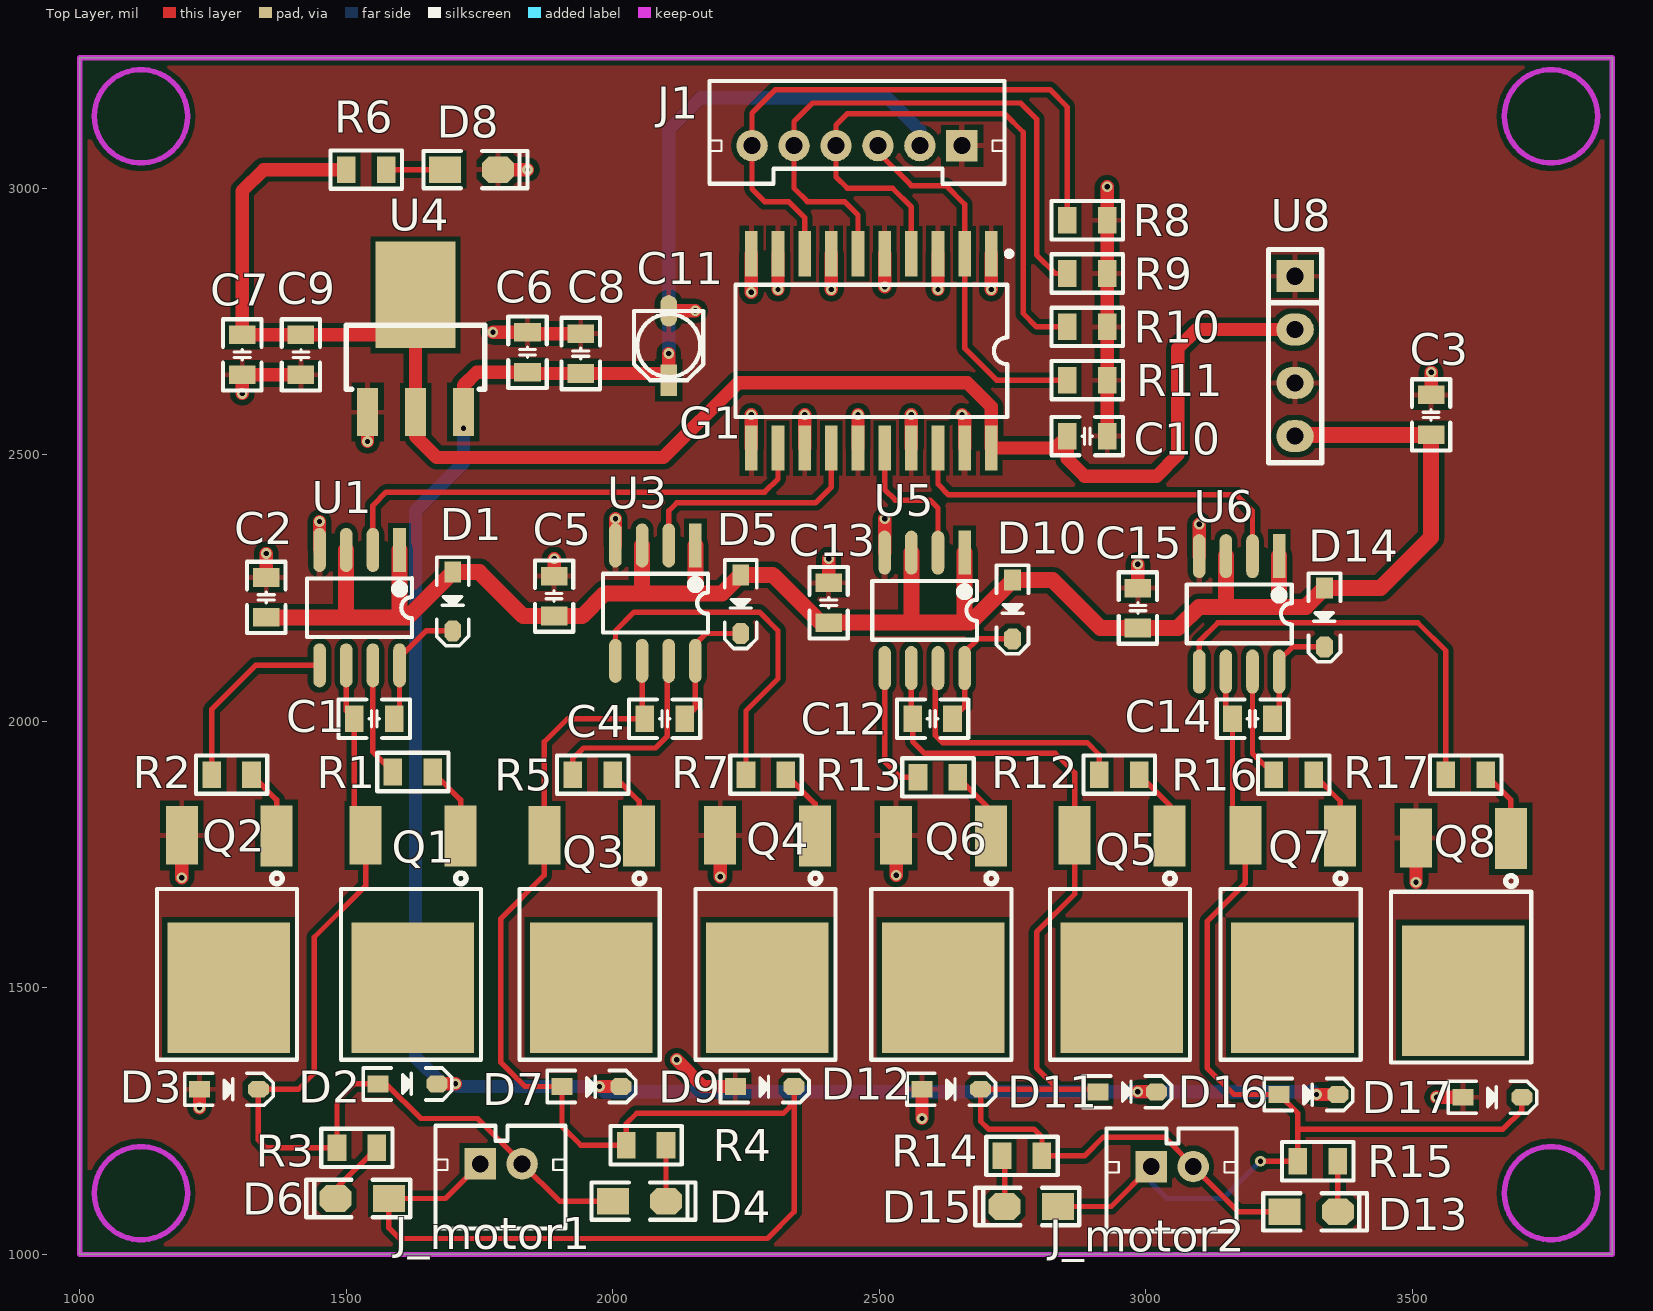
[diagram p0: Top Layer view]
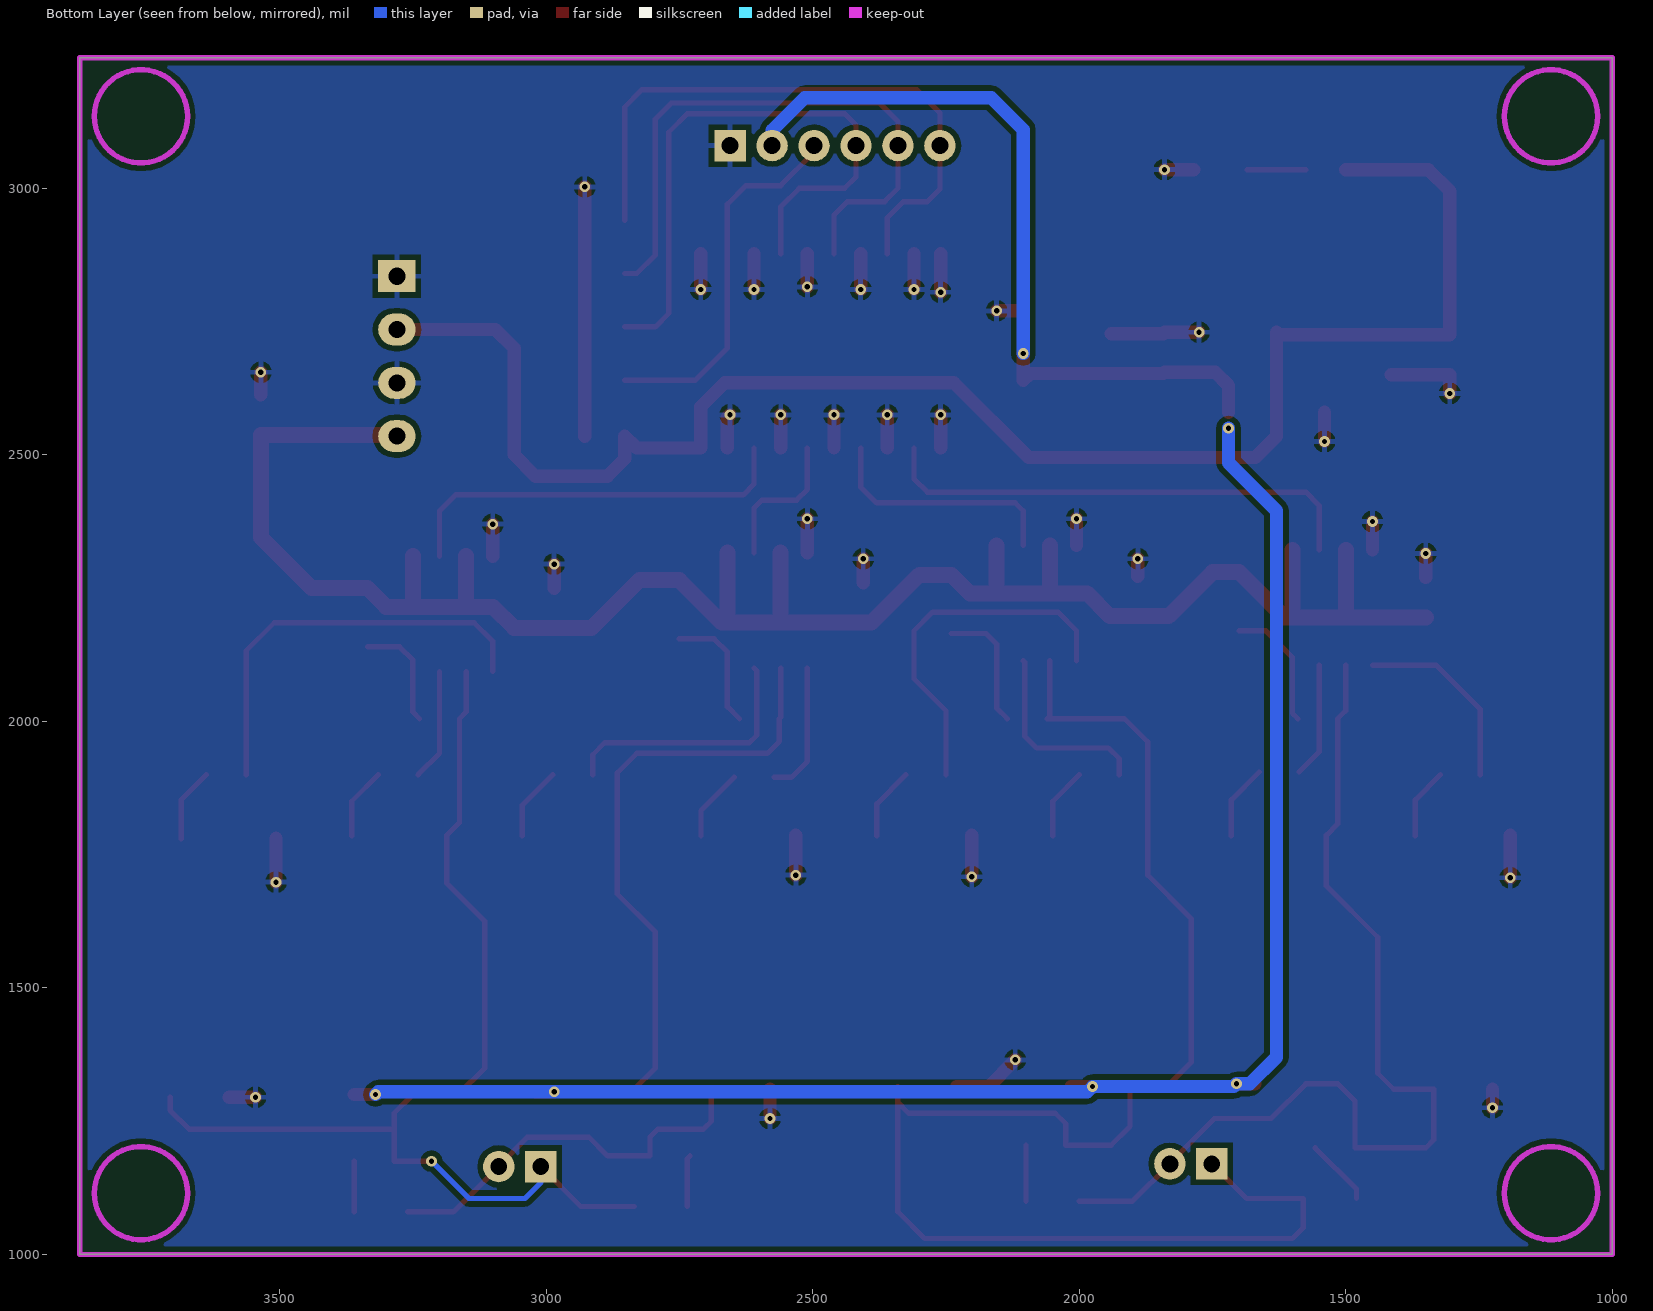
[diagram p1: Bottom Layer view, seen from below]
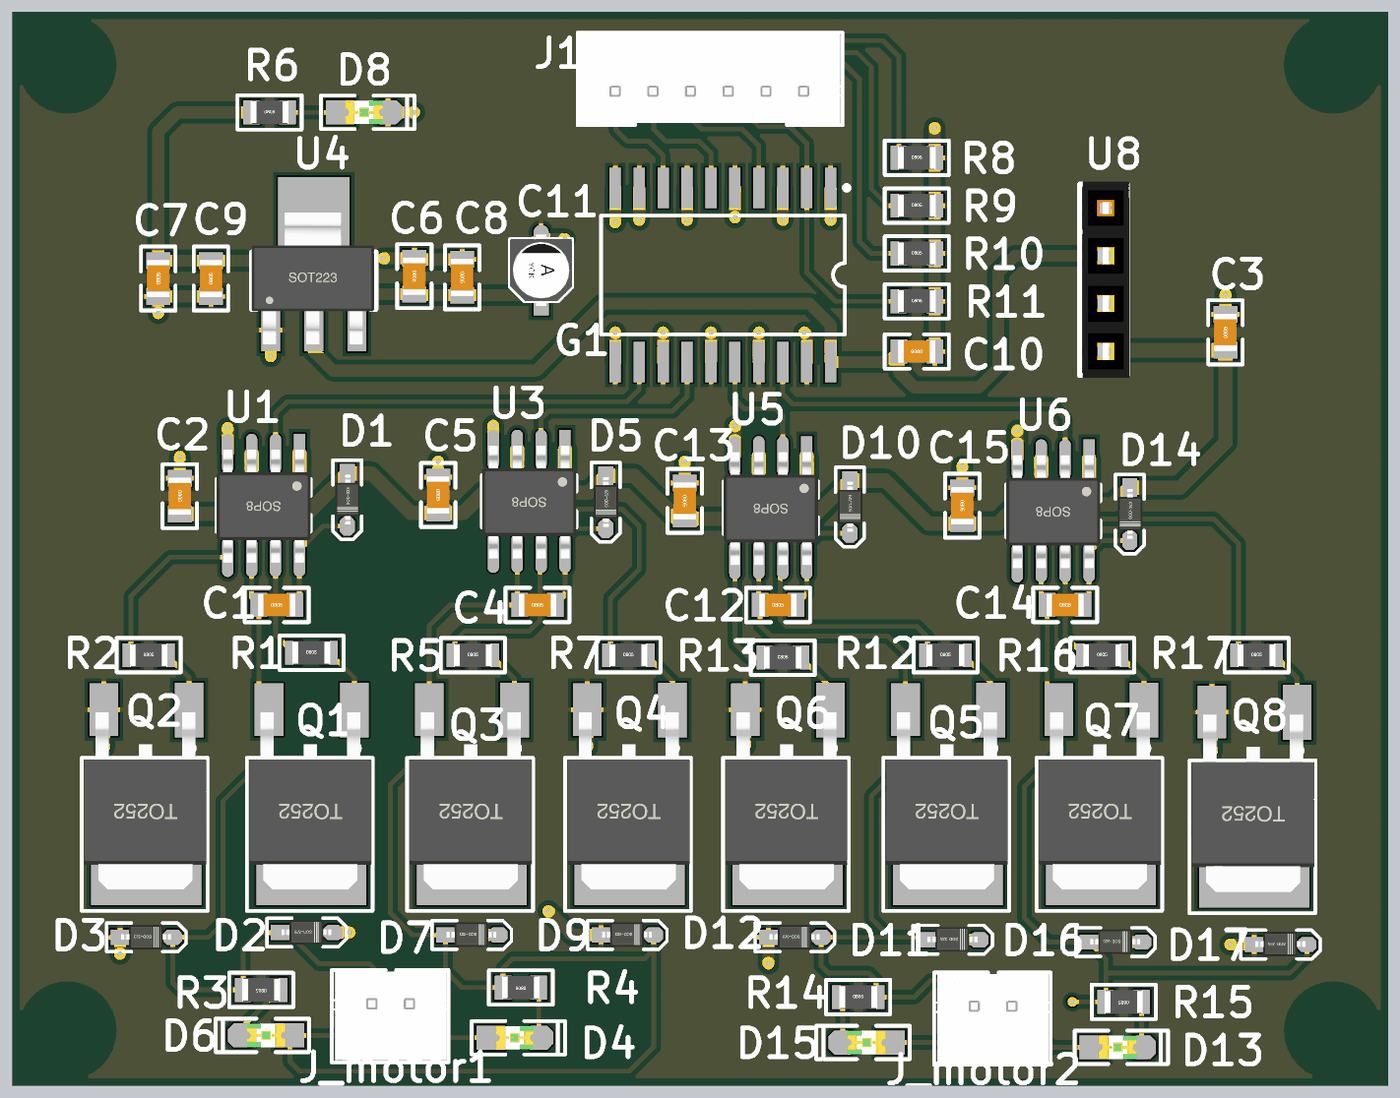
[diagram p2: 3D render of the assembled board from above, using the file's embedded part models]
# Altium PCB MISC82192.PcbDoc
Units mil, origin at the board's own origin, x right, y up, seen from the top; angles counter-clockwise.
Board outline 2875 x 2245 mil, 2 copper layers (Top Layer, Bottom Layer); 67 components, 41 nets, 192 pads, 41 vias.

## Layer stack, top to bottom (the 12.6 mil dielectric is the usual default, probably not edited)
Top Solder: solder mask 0.4, Solder Resist, Dk 3.5
Top Layer: signal copper 1.4
Dielectric 1: dielectric 12.6, FR-4, Dk 4.8
Bottom Layer: signal copper 1.4
Bottom Solder: solder mask 0.4, Solder Resist, Dk 3.5

## Board outline
1000,1000 3875,1000 3875,3245 1000,3245

## Design rules (kind name [scope] priority, off if disabled: settings)
Clearance [All] p1: gap=10
MinimumSolderMaskSliver [All] p1: minsoldermaskwidth=0
PolygonConnect [All] p1: connectstyle=Relief reliefconductorwidth=10 reliefentries=4 polygonreliefangle="90 Angle" airgapwidth=10
RoutingVias [All] p1: holewidth=28 width=50 viastyle="Through Hole" minholewidth=28 minwidth=50 maxholewidth=28 maxwidth=50
SilkToSilkClearance [All] p1: silktosilkclearance=0
SilkToSolderMaskClearance [IsPad] p1: minsilkscreentomaskgap=0 clearancetoexposedcopper=TRUE
SolderMaskExpansion [All] p1: expansion=4
Width [All] p1: maxlimit=1181.1 minlimit=10 preferedwidth=10
27 further rules are at their usual default settings.

## Components (designator, comment, footprint, x,y, rotation, side; value= is the part's Value field where it differs from the comment)
C1 "1.5UF" "C 0805_L" 1552.6,2005 r0 top
C2 "10UF" "C 0805_L" 1350,2232.6 r270 top
C3 "10uF" "C 0805_L" 3535,2575 r90 top
C4 "1.5UF" "C 0805_L" 2097.4,2005 r0 top
C5 "10UF" "C 0805_L" 1890,2235 r270 top
C6 "0.1UF" "C 0805_L" 1840,2692.4 r270 top
C7 "0.1UF" "C 0805_L" 1305,2687.6 r90 top
C8 "10UF" "C 0805_L" 1940,2690 r270 top
C9 "10UF" "C 0805_L" 1415,2687.6 r90 top
C10 "0.1UF" "C 0805_L" 2890,2535 r180 top
C11 "470UF" "CM A(3*5.4)" 2105,2705 r270 top
C12 "1.5UF" "C 0805_L" 2600,2005 r0 top
C13 "10UF" "C 0805_L" 2405,2222.6 r270 top
C14 "1.5UF" "C 0805_L" 3200,2005 r0 top
C15 "10UF" "C 0805_L" 2985,2212.6 r270 top
D1 "1N5819" SOD-323 1700,2225 r270 top
D2 "1N5819" SOD-323 1615.12,1320 r0 top
D3 "1N5819" SOD-323 1280,1310 r0 top
D4 "Red" "LED 0805G" 2050,1100 r0 top
D5 "1N5819" SOD-323 2240,2219.88 r270 top
D6 "Red" "LED 0805G" 1530,1105 r180 top
D7 "1N5819" SOD-323 1960,1315 r0 top
D8 "Red" "LED 0805G" 1735,3035 r0 top
D9 "1N5819" SOD-323 2285,1315 r0 top
D10 "1N5819" SOD-323 2750,2209.88 r270 top
D11 "1N5819" SOD-323 2965.12,1305 r0 top
D12 "1N5819" SOD-323 2635.12,1310 r0 top
D13 "Red" "LED 0805G" 3310,1080 r0 top
D14 "1N5819" SOD-323 3335,2194.88 r270 top
D15 "Red" "LED 0805G" 2785,1090 r180 top
D16 "1N5819" SOD-323 3305.12,1300 r0 top
D17 "1N5819" SOD-323 3650.12,1295 r0 top
G1 "SN74HC244DW" DW020 2485,2695 r180 top
J1 "CON6" PH2.0-6P 2654.96,3080 r180 top
J_motor1 "CON2" PH2.0-2P 1751.26,1170 r0 top
J_motor2 "CON2" PH2.0-2P 3010,1165 r0 top
Q1 "MOSFET-N4" TO252 1710,1785.35 r180 top
Q2 "MOSFET-N4" TO252 1365,1785.35 r180 top
Q3 "MOSFET-N4" TO252 2045,1785.35 r180 top
Q4 "MOSFET-N4" TO252 2375,1785.35 r180 top
Q5 "MOSFET-N4" TO252 3040,1785.35 r180 top
Q6 "MOSFET-N4" TO252 2705,1785.35 r180 top
Q7 "MOSFET-N4" TO252 3360,1785.35 r180 top
Q8 "MOSFET-N4" TO252 3680,1780.35 r180 top
R1 "20R" "R 0805_L" 1625,1905 r0 top
R2 "20R" "R 0805_L" 1285,1900 r0 top
R3 "1K" "R 0805_L" 1520,1200 r180 top
R4 "1K" "R 0805_L" 2062.6,1205 r180 top
R5 "20R" "R 0805_L" 1962.4,1900 r0 top
R6 "1K" "R 0805_L" 1537.6,3035 r0 top
R7 "20R" "R 0805_L" 2287.4,1900 r0 top
R8 "1K" "R 0805_L" 2890,2940 r0 top
R9 "1K" "R 0805_L" 2890,2840 r0 top
R10 "1K" "R 0805_L" 2890,2740 r0 top
R11 "1K" "R 0805_L" 2890,2640 r0 top
R12 "20R" "R 0805_L" 2950,1900 r0 top
R13 "20R" "R 0805_L" 2610,1895 r0 top
R14 "1K" "R 0805_L" 2767.6,1185 r0 top
R15 "1K" "R 0805_L" 3322.4,1175 r180 top
R16 "20R" "R 0805_L" 3277.4,1900 r0 top
R17 "20R" "R 0805_L" 3600,1900 r0 top
U1 "IR2104S" SOP8 1600,2321.54 r270 top
U3 "IR2104S" SOP8 2155,2330 r270 top
U4 "AMS1117" SOT223 1630,2580 r0 top
U5 "IR2104S" SOP8 2660,2316.54 r270 top
U6 "IR2104S" SOP8 3250,2310 r270 top
U8 "BL0512" Fe-HDR1X4/2.54-S 3280,2835 r0 top

## Footprints (in the part's own frame and the unit in brackets; to place one, negate y for a bottom-side part, rotate by r counter-clockwise, add the part's x,y. Pads: shape width x height; smd on the part's side, far side on the other; paste and mask are expansions set on the pad)
"C 0805_L" [mil] "无极性贴片电容"
  rect 35x50 smd: 1(-37.4,0) 2(37.4,0)
  silkscreen extent -67,-36 67,36, body extent -39,-24 39,24, height 20
"CM A(3*5.4)" [mm] "贴片电解电容，直径3mm，高5.4mm"
  rect 1.5x0.8 smd: 1(1.651,0)
  oval 1.5x0.8 smd: 2(-1.65,0)
  silkscreen extent -1.65,-1.65 1.65,1.65, body extent -1.9,-1.65 1.9,1.65, height 5.4
DW020 [mm] "Plastic Small Outline; 20 Leads; Body Width 7.5 mm"
  rect 0.6x2.15 smd: 1(-5.715,-4.625) 2(-4.445,-4.625) 3(-3.175,-4.625) 4(-1.905,-4.625) 5(-0.635,-4.625) 6(0.635,-4.625) 7(1.905,-4.625) 8(3.175,-4.625) 9(4.445,-4.625) 10(5.715,-4.625) 11(5.715,4.625) 12(4.445,4.625) 13(3.175,4.625) 14(1.905,4.625) 15(0.635,4.625) 16(-0.635,4.625) 17(-1.905,4.625) 18(-3.175,4.625) 19(-4.445,4.625) 20(-5.715,4.625)
  silkscreen extent -6.69,-4.75 6.47,3.15
Fe-HDR1X4/2.54-S [mil]
  rect 70x60 hole 32: 1(0,0)
  oval 70x60 hole 32: 2(0,-100) 3(0,-200) 4(0,-300)
  silkscreen extent -50,-350 50,50, body extent -44,-355 54,55, height 335
"LED 0805G" [mil] "绿色0805LED"
  rect 60x50 smd: 1(-50,0)
  oct 60x50 smd: 2(50,0)
  silkscreen extent -90,-35 105,35, body extent -39,-25 39,25, height 32
PH2.0-2P [mm]
  rect 1.5x1.5 hole 0.8: 1(0,0)
  round 1.5 hole 0.8: 2(2,0)
  silkscreen extent -2.13,-3.08 4.06,1.82, body extent -1.95,-2.97 3.95,1.73, height 6.01
PH2.0-6P [mm]
  rect 1.5x1.5 hole 0.8: 1(0,0)
  round 1.5 hole 0.8: 2(2,0) 3(4,0) 4(6,0) 5(8,0) 6(10,0)
  silkscreen extent -2.03,-3.08 12.03,1.82, body extent -1.91,-2.98 11.99,1.71, height 6.01
"R 0805_L" [mil] "1/8W贴片电阻"
  rect 35x50 smd: 1(-37.4,0) 2(37.4,0)
  silkscreen extent -67,-36 67,36, body extent -39,-25 39,25, height 20
SOD-323 [mm] "1.8x1.3X0.9mm（长宽高，不包括引脚）"
  rect 1x0.8 smd: 1(-1.4,0)
  oct 1x0.8 smd: 2(1.4,0)
  silkscreen extent -2.11,-0.76 2.11,0.76, body extent -1.34,-0.63 1.31,0.67, height 1
SOP8 [mm]
  rect 2.1x0.6 smd: 1(0,0)
  oval 2.1x0.6 smd: 2(0,-1.27) 3(0,-2.54) 4(0,-3.81) 5(5.5,-3.81) 6(5.5,-2.54) 7(5.5,-1.27) 8(5.5,0)
  silkscreen extent 1.35,-4.41 4.15,0.6, body extent -0.21,-4.4 5.8,0.6, height 1.9
SOT223 [mil]
  rect 40x90 smd: 1(-90,0) 2(0,0) 3(90,0)
  rect 150x200 smd: 2(0,220)
  silkscreen extent -130,43 130,163, body extent -130,-30 126,246, height 65
TO252 [mil] "252晶体管"
  rect 60x115 smd: 1(-4.55,0.23)
  rect 230x245 smd: 2(85,285.35)
  rect 60x110 smd: 3(173.45,-0.77)
  silkscreen extent -43,70 220,420, body extent -41,5 215,375, height 91

## Part data
C1 C2 C4 C5 C6 C7 C8 C9 C10 C12 C13 C14 C15: library part C, "SMD capacitor"
C3: library part CS_SMD, "SMD solid-state capacitor"
C11: library part CE_SMD, "SMD electrolytic capacitor"
D1 D2 D3 D5 D7 D9 D10 D11 D12 D14 D16 D17: "Schottky diode"
D4 D6 D8 D13 D15: library part LED-SMD, "SMD LED"
G1: "Octal Buffer and Line Driver with 3-State Outputs"
J1: library part PH2.0-6P
J_motor1 J_motor2: library part PH2.0-2P
Q1 Q2 Q3 Q4 Q5 Q6 Q7 Q8: "N-Channel MOSFET, Externally Terminated Substrate"
R1 R2 R3 R4 R5 R6 R7 R8 R9 R10 R11 R12 R13 R14 R15 R16 R17: library part R, "SMD resistor"
U1 U3 U5 U6: "High and Low Side Driver"
U4: "Three-terminal voltage regulator"
U8: library part "Female HDR1X4"

## Via types
v1: diameter 20, hole 10, Top Layer to Bottom Layer, 41 vias

## Nets (pads, with @x,y where several pads share a name; then routed paths per layer and width w, separated by ;. In a path a pad name is that pad's centre, name@x,y a point inside that pad or via, vN(x,y) a via of type N, cw(c..) or ccw(c..) an arc to the next point about the centre after c; other vN are vias at no path point)
5V: C7.2 C9.2 C10.2 G1.20 R6.1 U4.2 U8.2 | length 3120.4
  Top Layer w25: R6.1 1345,3035 1305,2995 C7.2 C9.2 1625,2725 1630,2730 1630,2580 1630,2535 1670,2495 2095,2495 2235,2635 2665,2635 2710,2590 G1.20 2830.51,2512.91 C10.2 2852.6,2492.4 2885,2460 3020,2460 3060,2500 3060,2700 3095,2735 U8.2
12V: C2.2 C3.1 C5.2 C13.2 C15.2 D1.1 D5.1 D10.1 D14.1 U1.1 U1.3 U3.1 U3.3 U5.1 U5.3 U6.1 U6.3 U8.4 | length 3810.7
  Top Layer w30: C2.2 1505,2195.2 ; U1.3 1500,2200.2 1505,2195.2 ; U1.1 1600,2195.2 ; U3.3 2055,2245 2060,2240 ; U3.1 2155,2245 2150,2240 ; U5.3 2560,2190.2 2565,2185.2 ; U5.1 2660,2195.39 2670.2,2185.2 ; U6.3 3150,2215 ; U6.1 3250,2215 ; U8.4 3282.6,2537.6 C3.1 3535,2345 3440,2250 D14.1 3300,2215 3250,2215 ; 1505,2195.2 1600,2195.2 ; 1600,2195.2 1615.08,2195.2 D1.1 1749.88,2280.12 1832.4,2197.6 C5.2 1942.6,2197.6 1985,2240 2060,2240 ; 2060,2240 2150,2240 ; 2150,2240 2205,2240 D5.1 2300,2275 2389.8,2185.2 C13.2 2565,2185.2 ; 2565,2185.2 2670.2,2185.2 ; 2670.2,2185.2 D10.1 2825,2265 2914.8,2175.2 C15.2 3060.2,2175.2 3100,2215 3150,2215 ; 3150,2215 3250,2215
BAT: C6.2 C8.2 C11.1 D2.2 D7.2 D11.2 D16.2 J1.2 U4.3 | length 4558.4
  Top Layer w25: D2.2 v1(1705,1320) ; U4.3 1720,2630 1745,2655 C6.2 1842.4,2652.6 C8.2 2092.4,2652.6 C11.1 v1(2105,2690) ; v1(1975,1315) D7.2 ; v1(2985,1305) D11.2 ; v1(3320,1300) D16.2
  Bottom Layer w25: v1(1720,2550) 1720,2485 1630,2395 1630,1370 1680,1320 v1(1705,1320) 1710,1315 v1(1975,1315) 1985,1305 v1(2985,1305) 3315,1305 v1(3320,1300) ; v1(2105,2690) 2105,3110 2165,3170 2515,3170 2576.22,3108.78 J1.2
GND: C2.1 C3.2 C5.1 C6.1 C7.1 C8.1 C9.1 C10.1 C11.2 C13.1 C15.1 D3.1 D8.2 D9.1 D12.1 D17.1 G1.1 G1.3 G1.5 G1.7 G1.9 G1.10 G1.11 G1.13 G1.15 G1.17 G1.19 J1.1 Q2.3 Q4.3 Q6.3 Q8.3 R8.2 R9.2 R10.2 R11.2 U1.4 U3.4 U4.1 U5.4 U6.4 U8.1 U8.3 | length 2675.7
  Top Layer w25: v1(1191.55,1706.55) Q2.3 ; v1(1224.88,1275.12) D3.1 ; v1(1305,2615) C7.1 C9.1 ; C2.1 v1(1350,2315) ; U1.4 v1(1450,2375) ; v1(1540,2525) U4.1 ; v1(1775.2,2729.8) C6.1 1842.4,2727.4 C8.1 ; D8.2 v1(1840,3035) ; C5.1 v1(1890,2305) ; U3.4 v1(2005,2380) ; C11.2 v1(2154.96,2769.96) ; v1(2120,1365) 2170,1315 D9.1 ; v1(2201.55,1708.45) Q4.3 ; G1.11 v1(2260,2575) ; v1(2260,2805) G1.10 ; v1(2310,2810) G1.9 ; G1.13 v1(2360,2575) ; C13.1 v1(2405,2305) ; v1(2410,2810) G1.7 ; G1.15 v1(2460,2575) ; U5.4 v1(2510,2380) ; v1(2510,2815) G1.5 ; v1(2531.55,1711.55) Q6.3 ; G1.17 v1(2560,2575) ; v1(2580,1255) D12.1 ; v1(2610,2810) G1.3 ; v1(2655,2575) 2660,2570 G1.19 ; v1(2710,2810) G1.1 ; C10.1 v1(2927.4,3002.6) ; C15.1 v1(2985,2295) ; U6.4 v1(3100,2370) ; v1(3506.55,1698.45) Q8.3 ; C3.2 v1(3535,2655) ; v1(3545,1295) D17.1
MOTORIN1: G1.16 U5.2 | length 275.9
  Top Layer w10: G1.16 2510,2435 2530,2415 2595,2415 2610,2400 U5.2
MOTORIN2: G1.18 U6.2 | length 763.6
  Top Layer w10: G1.18 2610,2445 2630,2425 3170,2425 3200,2395 U6.2
MOTORIN3: G1.14 U3.2 | length 461.6
  Top Layer w10: U3.2 2105,2395 2120,2410 2380,2410 2410,2440 G1.14
MOTORIN4: G1.12 U1.2 | length 922.1
  Top Layer w10: U1.2 1550,2405 1575,2430 2285,2430 2310,2455 G1.12
NetC1_2: C1.2 D1.2 U1.8 | length 239.8
  Top Layer w10: C1.2 1600,2015 U1.8 1600,2120 1649.88,2169.88 D1.2
NetC4_2: C4.2 D5.2 U3.8 | length 241.6
  Top Layer w10: C4.2 2155,2025.2 U3.8 2155,2145 2174.76,2164.76 D5.2
NetC12_2: C12.2 D10.2 U5.8 | length 234.6
  Top Layer w10: C12.2 2660,2027.6 U5.8 2660,2130 2684.76,2154.76 D10.2
NetC14_2: C14.2 D14.2 U6.8 | length 210.5
  Top Layer w10: C14.2 3250,2017.6 U6.8 3250,2115 3274.76,2139.76 D14.2
NetD4_2: D4.2 R4.1 | length 105
  Top Layer w10: D4.2 R4.1
NetD6_2: D6.2 R3.1 | length 127.1
  Top Layer w10: D6.2 1480,1122.6 R3.1
NetD8_1: D8.1 R6.2 | length 110
  Top Layer w10: R6.2 D8.1
NetD13_2: D13.2 R15.1 | length 95.1
  Top Layer w10: R15.1 3360,1174.8 D13.2
NetD15_2: D15.2 R14.1 | length 97
  Top Layer w10: R14.1 2735,1180.2 D15.2
NetQ1_1: Q1.1 R1.2 | length 141.5
  Top Layer w10: R1.2 1714.55,1852.84 Q1.1
NetQ2_1: Q2.1 R2.2 | length 134.4
  Top Layer w10: R2.2 1369.55,1852.84 Q2.1
NetQ3_1: Q3.1 R5.2 | length 135.5
  Top Layer w10: R5.2 2049.55,1850.25 Q3.1
NetQ4_1: Q4.1 R7.2 | length 137.6
  Top Layer w10: R7.2 2379.55,1845.25 Q4.1
NetQ5_1: Q5.1 R12.2 | length 138.5
  Top Layer w10: R12.2 3044.55,1842.84 Q5.1
NetQ6_1: Q6.1 R13.2 | length 135.6
  Top Layer w10: R13.2 2709.55,1832.84 Q6.1
NetQ7_1: Q7.1 R16.2 | length 135.5
  Top Layer w10: R16.2 3364.55,1850.25 Q7.1
NetQ8_1: Q8.1 R17.2 | length 139.4
  Top Layer w10: R17.2 3684.55,1852.84 Q8.1
NetR1_1: R1.1 U1.7 | length 215.6
  Top Layer w10: U1.7 1550,1942.59 R1.1
NetR2_1: R2.1 U1.5 | length 359.1
  Top Layer w10: R2.1 1247.6,2022.6 1330,2105 U1.5
NetR5_1: R5.1 U3.7 | length 367.1
  Top Layer w10: R5.1 1925,1930 1945,1950 2080,1950 2102.3,1972.3 2102.3,2110.77 U3.7
NetR7_1: R7.1 U3.5 | length 685.4
  Top Layer w10: U3.5 2005,2170 2040,2205 2275,2205 2310,2170 2310,2080 2250,2020 R7.1
NetR12_1: R12.1 U5.7 | length 488.5
  Top Layer w10: U5.7 2604.9,2094.9 2604.9,1973.79 2618.69,1960 2890,1960 2912.6,1937.4 R12.1
NetR13_1: R13.1 U5.5 | length 250
  Top Layer w10: U5.5 2510,1925 2540,1895 R13.1
NetR16_1: R16.1 U6.7 | length 210
  Top Layer w10: U6.7 3200,1940 R16.1
NetR17_1: R17.1 U6.5 | length 787.8
  Top Layer w10: U6.5 3100,2150 3135,2185 3510,2185 3562.6,2132.4 R17.1
OA1: C1.1 D2.1 D3.2 D4.1 J_motor1.2 Q1.3 R3.2 U1.6 | length 1896.6
  Top Layer w10: U1.6 1500,2020.2 C1.1 1515.2,1807.48 Q1.3 1536.55,1691.55 1440,1595 1440,1340 1410,1310 D3.2 1335.12,1214.88 1350,1200 R3.2 1482.6,1287.6 1515,1320 D2.1 1575,1320 1640,1255 1746.53,1255 1830,1171.53 J_motor1.2 1900,1100 D4.1
OA2: C12.1 D11.1 D12.2 D13.1 J_motor2.2 Q5.3 R14.2 U5.6 | length 2079.2
  Top Layer w10: U5.6 2560,2007.6 C12.1 2562.6,1962.4 2585,1940 2830,1940 2866.55,1903.45 Q5.3 2866.55,1676.55 2795,1605 2795,1350 2835,1310 ; D11.1 2905,1310 2835,1310 ; D13.1 3173.74,1080 J_motor2.2 3088.74,1166.53 3035.27,1220 2920,1220 2885,1185 R14.2 2805,1220 2790,1235 2705,1235 2690.24,1249.76 D12.2 2835,1310
OB1: C4.1 D6.1 D7.1 D9.2 J_motor1.1 Q3.3 R4.2 U3.6 | length 2944.5
  Top Layer w10: J_motor1.1 1686.26,1105 D6.1 1580,1050 1600,1030 2290,1030 2340.12,1080.12 2340.12,1285.12 ; U3.6 2055,2010 C4.1 1915,2005 1871.55,1961.55 Q3.3 1871.55,1711.55 1790,1630 1790,1360 1835,1315 D7.1 1904.88,1240.12 1940,1205 R4.2 2025.2,1245.2 2045,1265 2320,1265 2340.12,1285.12 ; D9.2 2340.12,1285.12
OB2: C14.1 D15.1 D16.1 D17.2 J_motor2.1 Q7.3 R15.2 U6.6 | length 2095.5
  Top Layer w10: D15.1 2935,1090 J_motor2.1 ; U6.6 3150,2017.6 C14.1 3162.6,1810.08 Q7.3 3186.55,1696.55 3115,1625 3115,1350 3165,1300 D16.1 3285,1265 3285,1235 ; v1(3215,1175) R15.2 3285,1235 ; D17.2 3705.24,1270.24 3670,1235 3285,1235
  Bottom Layer w10: J_motor2.1 3010,1135 3040,1105 3145,1105 v1(3215,1175)
PWM1: G1.8 J1.6 R8.1 | length 1166.8
  Top Layer w10: G1.8 2360,2945 2330,2975 2285,2975 2261.26,2998.74 J1.6 2261.26,3141.26 2305,3185 2820,3185 2852.6,3152.4 R8.1
PWM2: G1.6 J1.5 R9.1 | length 1147.6
  Top Layer w10: G1.6 2460,2950 2435,2975 2365,2975 2340,3000 J1.5 2340,3125 2375,3160 2765,3160 2795,3130 2795,2875 2830,2840 R9.1
PWM3: G1.4 J1.4 R10.1 | length 1157.5
  Top Layer w10: G1.4 2560,2965 2525,3000 2440,3000 2418.74,3021.26 J1.4 2418.74,3118.74 2440,3140 2735,3140 2770,3105 2770,2765 2795,2740 R10.1
PWM4: G1.2 J1.3 R11.1 | length 702.8
  Top Layer w10: J1.3 2497.48,3067.52 2560,3005 2625,3005 2660,2970 G1.2 2660,2700 2720,2640 R11.1
pads on no net: Q1.2 Q2.2 Q3.2 Q4.2 Q5.2 Q6.2 Q7.2 Q8.2

## Polygon pours and split planes (outlines as drawn)
GND on Top Layer "D" (solid, remove dead copper, pour order 0): 615,3390 620,3395 4030,3395 4030,870 4075,825 4050,800 590,800
GND on Bottom Layer "D" (solid, remove dead copper, pour order 2): 755,3385 4035,3385 4105,3315 4010,3220 4010,835 760,835 740,815

## Keep-outs
Keep-Out Layer:
  circle w10: c3760,3135 r87.46
  circle w10: c3760,1115 r87.46
  circle w10: c1115,1115 r87.46
  circle w10: c1115,3135 r87.46
  lines w10: 1000,1000 1000,3245 3875,3245 3875,1000 1000,1000